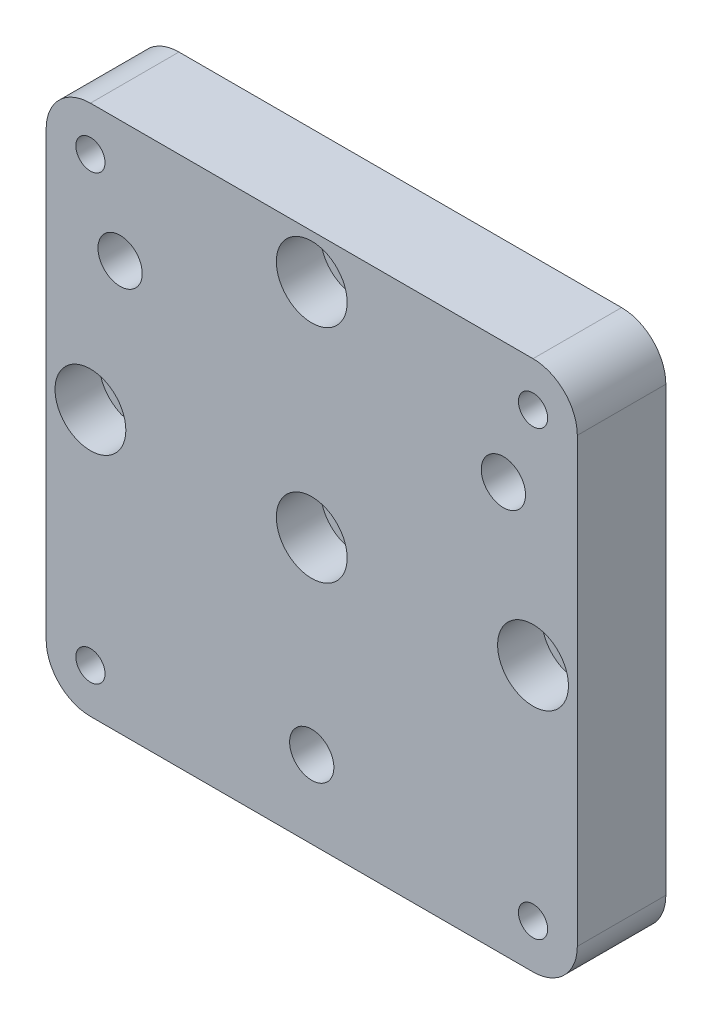
from build123d import *

# Parameters (mm, degrees)
SKETCH1_W             = 60
SKETCH1_H             = 60
BOSS_EXTRUDE1_DEPTH   = 10
FILLET1_R             = 5
M6_TAPPED_HOLE1_D     = 5
M6_TAPPED_HOLE1_DEPTH = 15
M6_TAPPED_HOLE1_TIP   = 1.502151548
SKETCH8_R             = 2.1
CUT_EXTRUDE1_DEPTH    = 51.336896077
SKETCH9_R             = 4
CUT_EXTRUDE2_DEPTH    = 5
M4_TAPPED_HOLE1_D     = 3.3
M4_TAPPED_HOLE2_D     = 3.3
SKETCH15_R            = 4
CUT_EXTRUDE3_DEPTH    = 5
SKETCH16_R            = 2.1
CUT_EXTRUDE4_DEPTH    = 51.336896077


with BuildPart() as part:
    # Sketch1 → Boss-Extrude1 (new body)
    with BuildSketch(Plane.XY):
        with Locations((9.163798419, 0)):
            Rectangle(SKETCH1_W, SKETCH1_H)
    extrude(amount=BOSS_EXTRUDE1_DEPTH)

    # Fillet1
    fillet1_edges = [part.edges().sort_by_distance(p)[0] for p in [
        (-20.836201581, 30, 5),
        (39.163798419, 30, 5),
        (39.163798419, -30, 5),
        (-20.836201581, -30, 5),
    ]]
    fillet(fillet1_edges, radius=FILLET1_R)

    # M6 Tapped Hole1
    with Locations(Plane.XY.offset(10)):
        with Locations((9.163798419, -21.25), (30.814433514, 16.25), (-12.486836675, 16.25)):
            Hole(M6_TAPPED_HOLE1_D / 2, depth=M6_TAPPED_HOLE1_DEPTH)
            with Locations((0, 0, -(M6_TAPPED_HOLE1_DEPTH + M6_TAPPED_HOLE1_TIP / 2))):  # 118° drill point
                Cone(0, M6_TAPPED_HOLE1_D / 2, M6_TAPPED_HOLE1_TIP, mode=Mode.SUBTRACT)

    # Sketch8 → Cut-Extrude1 (cut, through all)
    with BuildSketch(Plane.XY.offset(10)):
        with Locations((9.163798419, 25)):
            Circle(SKETCH8_R)
        with Locations((34.163798419, 0)):
            Circle(SKETCH8_R)
        with Locations((-15.836201581, 0)):
            Circle(SKETCH8_R)
    extrude(amount=-CUT_EXTRUDE1_DEPTH, mode=Mode.SUBTRACT)

    # Sketch9 → Cut-Extrude2 (cut)
    with BuildSketch(Plane.XY.offset(10)):
        with Locations((-15.836201581, 0)):
            Circle(SKETCH9_R)
        with Locations((9.163798419, 25)):
            Circle(SKETCH9_R)
        with Locations((34.163798419, 0)):
            Circle(SKETCH9_R)
    extrude(amount=-CUT_EXTRUDE2_DEPTH, mode=Mode.SUBTRACT)

    # M4 Tapped Hole1 (through all)
    with Locations(Plane.XY.offset(10)):
        with Locations((-15.836201581, -25), (34.163798419, -25), (34.163798419, 25), (-15.836201581, 25)):
            Hole(M4_TAPPED_HOLE1_D / 2)

    # M4 Tapped Hole2 (through all)
    with Locations(Plane.XY.offset(10)):
        with Locations((9.163798419, 0)):
            Hole(M4_TAPPED_HOLE2_D / 2)

    # Sketch15 → Cut-Extrude3 (cut)
    with BuildSketch(Plane.XY.offset(10)):
        with Locations((9.163798419, 0)):
            Circle(SKETCH15_R)
    extrude(amount=-CUT_EXTRUDE3_DEPTH, mode=Mode.SUBTRACT)

    # Sketch16 → Cut-Extrude4 (cut, through all)
    with BuildSketch(Plane.XY.offset(10)):
        with Locations((9.163798419, 0)):
            Circle(SKETCH16_R)
    extrude(amount=-CUT_EXTRUDE4_DEPTH, mode=Mode.SUBTRACT)


solid = part.part
